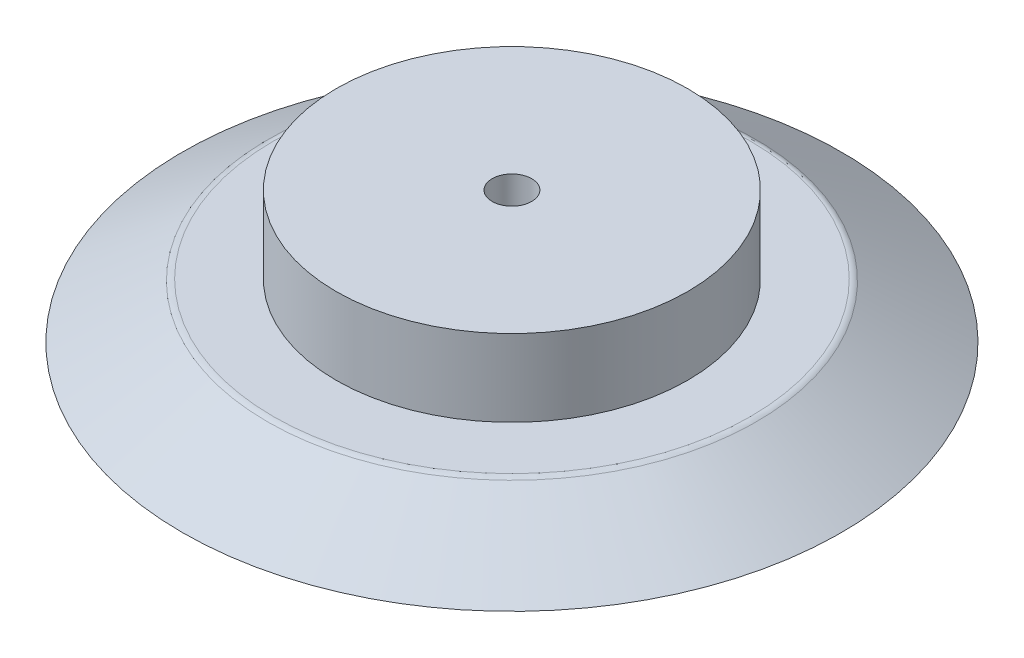
from build123d import *

# Parameters (mm, degrees)
CLEARANCE_HOLE_FOR_M1_62_D = 1.8


with BuildPart() as part:
    # Sketch1 → Revolution1 (revolve)
    with BuildSketch(Plane.XY, mode=Mode.PRIVATE) as revolution1_sk:
        with BuildLine():
            Line((0, -15.453508628), (-15, -15.453508628))
            Line((-15, -15.453508628), (-11.121601357, -13.029509476))
            ThreePointArc((-11.121601357, -13.029509476), (-10.994443143, -12.972884255), (-10.856601887, -12.953508628))
            Line((-10.856601887, -12.953508628), (-8, -12.953508628))
            Line((-8, -12.953508628), (-8, -11.453508628))
            Line((-8, -11.453508628), (-8, -9.453508628))
            Line((-8, -9.453508628), (0, -9.453508628))
            Line((0, -9.453508628), (0, -15.453508628))
        make_face()
    revolve(revolution1_sk.sketch.rotate(Axis((0, 20.85946169, 0), (0, -1, 0)), 270), axis=Axis((0, 20.85946169, 0), (0, -1, 0)))

    # Clearance hole for M1.62 (through all)
    with Locations(Plane(origin=(0, -15.453508628, 0), x_dir=(-1, 0, 0), z_dir=(0, -1, 0))):
        with Locations((0, 0)):
            Hole(CLEARANCE_HOLE_FOR_M1_62_D / 2)


solid = part.part
